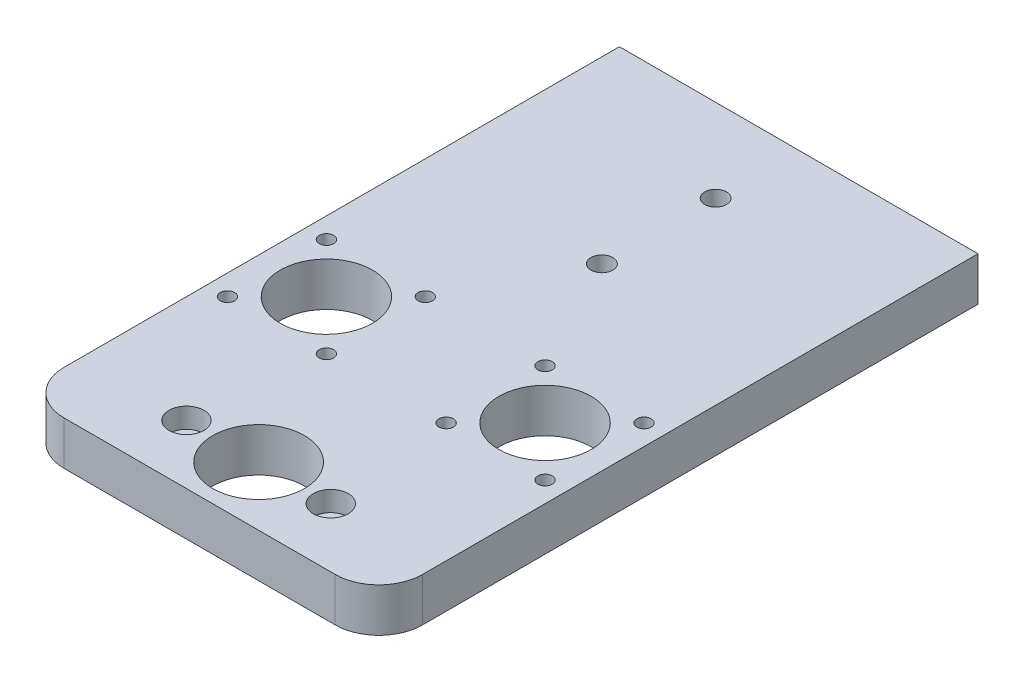
SolidWorks part; units mm, degrees
material "6061铝"
ref_plane "前视基准面" through (0, 0, 0) normal (0, 0, 1) x (1, 0, 0)
ref_plane "上视基准面" through (0, 0, 0) normal (0, 1, 0) x (1, 0, 0)
ref_plane "右视基准面" through (0, 0, 0) normal (1, 0, 0) x (0, 0, -1)
sketch "草图1" plane through (0, 0, 0) normal (0, 1, 0) x (1, 0, 0)
  line L1 (-41, 68.5) -> (41, 68.5)
  line L2 (-41, 68.5) -> (-41, -68.5)
  line L3 (-41, -68.5) -> (41, -68.5)
  line L4 (41, 68.5) -> (41, -68.5)
  line L5 (-41, 68.5) -> (41, -68.5) construction
  line L6 (-41, -68.5) -> (41, 68.5) construction
  point P0 (0, 0)
  dimension "D1" = 82
  dimension "D2" = 137
extrude "凸台-拉伸1" add sketch "草图1" along normal blind 10
sketch "草图4" plane through (0, 10, 0) normal (0, 1, 0) x (1, 0, 0)
  line L1 (-41, -68.5) -> (41, -68.5) construction
  circle A0 centre (0, -55) radius 10.5
  dimension "D1" = 21
  dimension "D2" = 13.5
extrude "切除-拉伸3" cut sketch "草图4" against normal through all
fillet "圆角9" radius 10 2 edges at (-41, 5, 68.5) (41, 5, 68.5)
hole_wizard "打孔尺寸(%根据)开槽圆柱头螺钉的类型2" positions "草图34" profile "草图35" counterbore size "M4" standard "GB" end condition through all
sketch "草图34" plane through (0, 10, 0) normal (0, 1, 0) x (1, 0, 0)
  line L0 (-16.5, -55) -> (16.5, -55) construction
  line L3 (0, 0) -> (0, -55) construction
  circle A0 centre (0, -55) radius 10.5 construction
  point P0 (-16.5, -55)
  point P2 (16.5, -55)
  dimension "D2" = 33
  dimension "D3" = 0
sketch "草图35" plane through (-16.5, 10, 55) normal (1, 0, 0) x (0, 0, 1)
  line L0 (0, 0) -> (0, 10)
  line L1 (0, 10) -> (2.15, 10)
  line L3 (2.15, 10) -> (2.15, 4.6)
  line L4 (2.15, 4.6) -> (4, 4.6)
  line L5 (4, 4.6) -> (4, 0)
  line L7 (4, 0) -> (0, 0)
  line L11 (0, -6.35) -> (0, 107.95) construction
  dimension "通孔孔直径" = 4.3
  dimension "通孔孔深度" = 10
  dimension "柱形沉头孔直径" = 8
  dimension "柱形沉头孔深度" = 4.6
hole_wizard "M4 螺纹孔2" positions "草图49" profile "草图50" tap size "M4" standard "GB"
sketch "草图49" plane through (0, 0, -68.5) normal (0, 0, -1) x (-1, 0, 0)
  line L0 (-15, 5) -> (15, 5) construction
  line L5 (0, 5) -> (0, 0) construction
  line L6 (15, 5) -> (41, 5) construction
  line L7 (41, 10) -> (41, 0) construction
  point P0 (-15, 5)
  point P2 (15, 5)
  dimension "D1" = 30
sketch "草图50" plane through (15, 5, -68.5) normal (1, 0, 0) x (0, 1, 0)
  line L0 (0, 0) -> (0, 19.4914)
  line L1 (0, 19.4914) -> (1.65, 18.5)
  line L2 (1.65, 18.5) -> (1.65, 0)
  line L5 (1.65, 0) -> (0, 0)
  line L10 (0, 19.4914) -> (-1.65, 18.5) construction
  line L11 (0, -6.35) -> (0, 107.95) construction
  dimension "螺纹孔钻头直径" = 3.3
  dimension "螺纹孔钻头深度" = 18.5
  dimension "导头角度" = 118
cosmetic thread "孔螺蚊线3" parameters "D1"=15, "D2"=4
cosmetic thread "孔螺蚊线4" parameters "D1"=15, "D2"=4
hole_wizard "大小mm 暗销孔2" positions "草图55" profile "草图57" hole size "Ø20.0" standard "GB" end condition through all
sketch "草图55" plane through (0, 10, 0) normal (0, 1, 0) x (1, 0, 0)
  line L0 (0, 0) -> (0, 50.6661) construction
  line L2 (-31, -68.5) -> (31, -68.5) construction
  point P0 (-25, -14.5)
  point P7 (25, -14.5)
  dimension "D1" = 50
  dimension "D2" = 54
sketch "草图57" plane through (-25, 10, 14.5) normal (1, 0, 0) x (0, 0, 1)
  line L0 (0, 0) -> (0, 10)
  line L1 (0, 10) -> (10.55, 10)
  line L2 (10.55, 10) -> (10.55, 0)
  line L5 (10.55, 0) -> (0, 0)
  line L11 (0, -6.35) -> (0, 107.95) construction
  dimension "通孔孔直径" = 21.1
  dimension "通孔孔深度" = 10
hole_wizard "M4 螺纹孔3" positions "草图58" profile "草图60" tap size "M4" standard "GB" end condition through all
sketch "草图58" plane through (0, 0, 0) normal (0, -1, 0) x (-1, 0, 0)
  point P15 (-13.6863, -3.1863)
  point P18 (-36.3137, -3.1863)
  point P21 (-36.3137, -25.8137)
  point P24 (-13.6863, -25.8137)
sketch "草图60" plane through (13.6863, 0, 3.1863) normal (1, 0, 0) x (0, 0, -1)
  line L0 (0, 0) -> (0, 10)
  line L1 (0, 10) -> (1.65, 10)
  line L2 (1.65, 10) -> (1.65, 0)
  line L5 (1.65, 0) -> (0, 0)
  line L11 (0, -6.35) -> (0, 107.95) construction
  dimension "通孔螺纹孔钻头直径" = 3.3
  dimension "通孔螺纹孔钻头深度" = 10
cosmetic thread "孔螺蚊线9" parameters "D2"=4
cosmetic thread "孔螺蚊线10" parameters "D2"=4
cosmetic thread "孔螺蚊线11" parameters "D2"=4
cosmetic thread "孔螺蚊线12" parameters "D2"=4
mirror "镜向2" about plane through (0, 0, 0) normal (1, 0, 0) of "M4 螺纹孔3"
hole_wizard "大小mm 暗销孔2" positions "草图61" profile "草图63" hole size "Ø5.0" standard "GB"
sketch "草图61" plane through (0, 0, -68.5) normal (0, 0, -1) x (-1, 0, 0)
  line L0 (-15, 5) -> (-50.274, 5) construction
  line L1 (0, 0) -> (0, 27.1576) construction
  point P9 (-32.5, 5)
  point P16 (32.5, 5)
  dimension "D1" = 65
sketch "草图63" plane through (-32.5, 5, -68.5) normal (1, 0, 0) x (0, 1, 0)
  line L0 (0, 0) -> (0, 11.6022)
  line L1 (0, 11.6022) -> (2.5, 10.1)
  line L2 (2.5, 10.1) -> (2.5, 0)
  line L5 (2.5, 0) -> (0, 0)
  line L10 (0, 11.6022) -> (-2.5, 10.1) construction
  line L11 (0, -6.35) -> (0, 107.95) construction
  dimension "孔直径" = 5
  dimension "孔深度" = 10.1
  dimension "导头角度" = 118
hole_wizard "M6 螺纹孔1" positions "草图64" profile "草图65" tap size "M6" standard "GB"
sketch "草图64" plane through (0, 10, 0) normal (0, 1, 0) x (1, 0, 0)
  line L0 (41, 68.5) -> (-41, 68.5) construction
  point P0 (0, 49.5)
  dimension "D1" = 19
sketch "草图65" plane through (0, 10, -49.5) normal (1, 0, 0) x (0, 0, 1)
  line L0 (0, 0) -> (0, 16.5022)
  line L1 (0, 16.5022) -> (2.5, 15)
  line L2 (2.5, 15) -> (2.5, 0)
  line L5 (2.5, 0) -> (0, 0)
  line L10 (0, 16.5022) -> (-2.5, 15) construction
  line L11 (0, -6.35) -> (0, 107.95) construction
  dimension "螺纹孔钻头直径" = 5
  dimension "螺纹孔钻头深度" = 15
  dimension "导头角度" = 118
cosmetic thread "孔螺蚊线13" parameters "D1"=10, "D2"=6
hole_wizard "M6 螺纹孔4" positions "草图70" profile "草图71" tap size "M6" standard "GB" end condition through all
sketch "草图70" plane through (0, 10, 0) normal (0, 1, 0) x (1, 0, 0)
  point P0 (0, 23.5)
sketch "草图71" plane through (0, 10, -23.5) normal (1, 0, 0) x (0, 0, 1)
  line L0 (0, 0) -> (0, 10)
  line L1 (0, 10) -> (2.5, 10)
  line L2 (2.5, 10) -> (2.5, 0)
  line L5 (2.5, 0) -> (0, 0)
  line L11 (0, -6.35) -> (0, 107.95) construction
  dimension "通孔螺纹孔钻头直径" = 5
  dimension "通孔螺纹孔钻头深度" = 10
cosmetic thread "孔螺蚊线16" parameters "D2"=6
